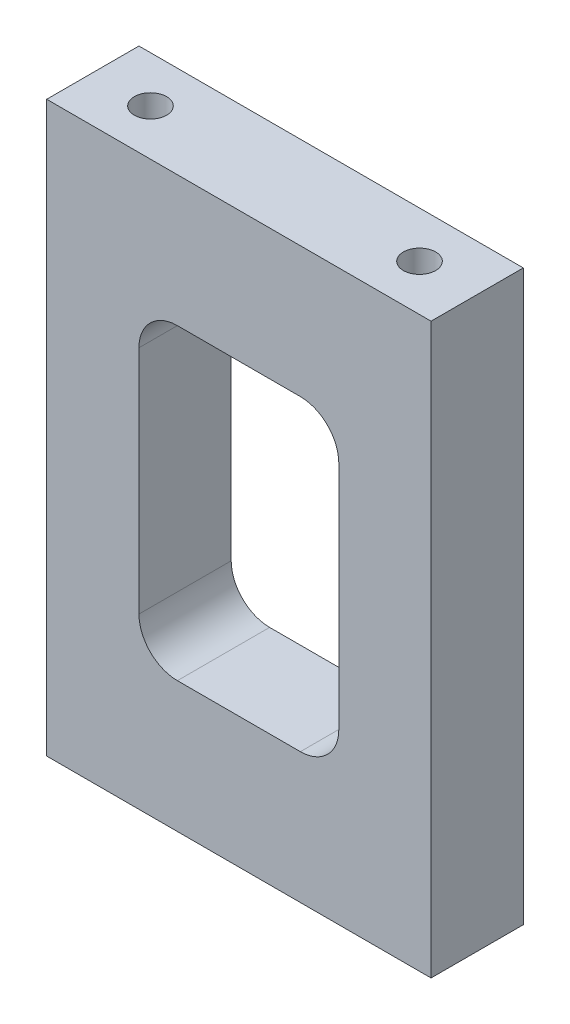
SolidWorks part; units mm, degrees
ref_plane "前视基准面" through (0, 0, 0) normal (0, 0, 1) x (1, 0, 0)
ref_plane "上视基准面" through (0, 0, 0) normal (0, 1, 0) x (1, 0, 0)
ref_plane "右视基准面" through (0, 0, 0) normal (1, 0, 0) x (0, 0, -1)
sketch "草图1" plane through (0, 0, 0) normal (0, 0, 1) x (1, 0, 0)
  line L1 (-25, -37) -> (25, -37)
  line L2 (-25, -37) -> (-25, 37)
  line L3 (-25, 37) -> (25, 37)
  line L4 (25, -37) -> (25, 37)
  line L5 (-25, -37) -> (25, 37) construction
  line L6 (-25, 37) -> (25, -37) construction
  point P0 (0, 0)
  dimension "D1" = 50
  dimension "D2" = 74
extrude "凸台-拉伸1" add sketch "草图1" along normal mid plane 12
sketch "草图4" plane through (0, -37, 0) normal (0, -1, 0) x (-1, 0, 0)
  point P0 (17.5, 0)
  point P3 (-17.5, 0)
hole_wizard "M5 螺纹孔1" positions "草图4" profile "草图3" tap size "M5" standard "GB"
sketch "草图3" plane through (-17.5, -37, 0) normal (1, 0, 0) x (0, 0, -1)
  line L0 (0, 0) -> (0, 13.6618)
  line L1 (0, 13.6618) -> (2.1, 12.4)
  line L2 (2.1, 12.4) -> (2.1, 0)
  line L5 (2.1, 0) -> (0, 0)
  line L10 (0, 13.6618) -> (-2.1, 12.4) construction
  line L11 (0, -6.35) -> (0, 107.95) construction
  dimension "螺纹孔钻头直径" = 4.2
  dimension "螺纹孔钻头深度" = 12.4
  dimension "导头角度" = 118
cosmetic thread "孔螺纹线1" parameters "D1"=10, "D2"=5
cosmetic thread "孔螺纹线2" parameters "D1"=10, "D2"=5
mirror "镜向1" about plane through (0, 0, 0) normal (0, 1, 0) of "M5 螺纹孔1"
sketch "草图5" plane through (0, 0, 6) normal (0, 0, 1) x (1, 0, 0)
  line L0 (25, -37) -> (25, 37) construction
  line L1 (-8, -20) -> (8, -20)
  line L2 (-13, -15) -> (-13, 15)
  line L3 (-8, 20) -> (8, 20)
  line L4 (13, -15) -> (13, 15)
  line L5 (-13, -20) -> (13, 20) construction
  line L6 (-13, 20) -> (13, -20) construction
  arc A0 (8, -20) -> (13, -15) centre (8, -15) ccw
  arc A1 (-13, 15) -> (-8, 20) centre (-8, 15) cw
  arc A2 (-8, -20) -> (-13, -15) centre (-8, -15) cw
  arc A3 (8, 20) -> (13, 15) centre (8, 15) cw
  point P0 (0, 0)
  dimension "D3" = 5
  dimension "D1" = 12
  dimension "D2" = 40
extrude "切除-拉伸1" cut sketch "草图5" against normal through all
